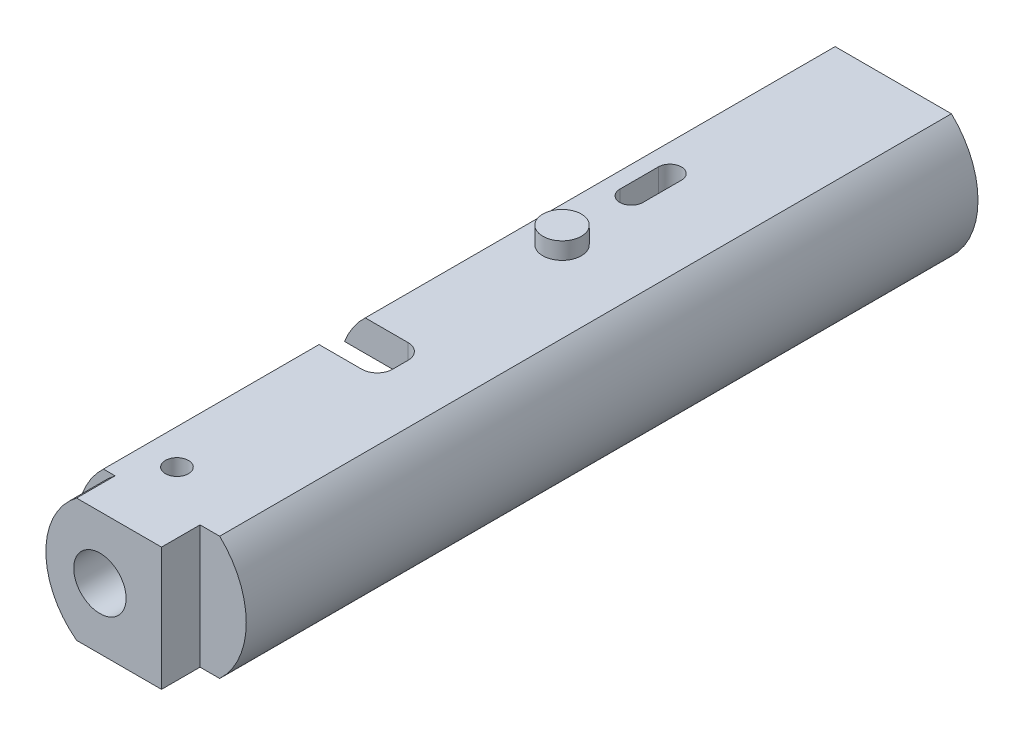
from build123d import *

# Parameters (mm, degrees)
SKETCH1_R                  = 11
BOSS_EXTRUDE1_DEPTH        = 100
CUT_EXTRUDE1_DEPTH         = 102.202766761
SKETCH3_R                  = 2
CUT_EXTRUDE2_DEPTH         = 60
CUT_EXTRUDE3_START         = -15
SKETCH4_W                  = 13.898015679
SKETCH4_H                  = 8
CUT_EXTRUDE3_DEPTH         = 65
CUT_EXTRUDE4_DEPTH         = 102.867561078
CUT_EXTRUDE4_DEPTH_BACK    = 102.867561078
SKETCH5_W                  = 12
SKETCH5_H                  = 10
M8_TAPPED_HOLE1_D          = 6.8
M8_TAPPED_HOLE1_DEPTH      = 10
M8_TAPPED_HOLE1_TIP        = 2.042926105
CUT_EXTRUDE5_START         = -3
SKETCH8_R                  = 1.5
CUT_EXTRUDE5_DEPTH         = 105.867561078
CUT_EXTRUDE6_DEPTH         = 102.867561078
CUT_EXTRUDE7_DEPTH         = 102.316336294
CUT_EXTRUDE7_DEPTH_BACK    = 102.316336294
M12X1_5_TAPPED_HOLE1_D     = 10.5
M12X1_5_TAPPED_HOLE1_DEPTH = 19.5
M12X1_5_TAPPED_HOLE1_TIP   = 3.15451825
SKETCH12_R                 = 2.5
BOSS_EXTRUDE2_DEPTH        = 2.2
BOSS_EXTRUDE3_START        = 2.2
SKETCH13_R                 = 2.5
BOSS_EXTRUDE3_DEPTH        = 2.2
SKETCH14_R                 = 3.5
CUT_EXTRUDE8_DEPTH         = 40
SKETCH15_R                 = 14.729549922
SKETCH15_R_2               = 10.018203868
CUT_EXTRUDE9_DEPTH         = 5


with BuildPart() as part:
    # Sketch1 → Boss-Extrude1 (new body)
    with BuildSketch(Plane.XY):
        Circle(SKETCH1_R)
    extrude(amount=BOSS_EXTRUDE1_DEPTH)

    # Sketch2 → Cut-Extrude1 (cut, through all)
    with BuildSketch(Plane.XY.offset(100)):
        with BuildLine():
            Line((-7.549834435, 8), (7.549834435, 8))
            ThreePointArc((7.549834435, 8), (0, 11), (-7.549834435, 8))
        make_face()
        with BuildLine():
            Line((-7.549834435, -8), (7.549834435, -8))
            ThreePointArc((7.549834435, -8), (0, -11), (-7.549834435, -8))
        make_face()
    extrude(amount=-CUT_EXTRUDE1_DEPTH, mode=Mode.SUBTRACT)

    # Sketch3 → Cut-Extrude2 (cut)
    with BuildSketch(Plane.XY.offset(100)):
        with Locations((-3, 0)):
            Circle(SKETCH3_R)
    extrude(amount=-CUT_EXTRUDE2_DEPTH, mode=Mode.SUBTRACT)

    # Sketch4 → Cut-Extrude3 (cut)
    with BuildSketch(Plane.XY.offset(100).offset(CUT_EXTRUDE3_START)):
        with Locations((-5.94900784, 0)):
            Rectangle(SKETCH4_W, SKETCH4_H)
    extrude(amount=-CUT_EXTRUDE3_DEPTH, mode=Mode.SUBTRACT)

    # Sketch5 → Cut-Extrude4 (cut, two sides: drawn at the far end of the back side and taken through both)
    with BuildSketch(Plane(origin=(0, -8, 0), x_dir=(-1, 0, 0), z_dir=(0, -1, 0)).offset(-CUT_EXTRUDE4_DEPTH_BACK)):
        with Locations((-11, -100)):
            Rectangle(SKETCH5_W, SKETCH5_H)
    extrude(amount=CUT_EXTRUDE4_DEPTH + CUT_EXTRUDE4_DEPTH_BACK, mode=Mode.SUBTRACT)

    # M8 Tapped Hole1
    with Locations(Plane(origin=(-3, -0.07100101, 100), x_dir=(1, 0, 0), z_dir=(0, 0, 1))):
        with Locations((0, 0)):
            Hole(M8_TAPPED_HOLE1_D / 2, depth=M8_TAPPED_HOLE1_DEPTH)
            with Locations((0, 0, -(M8_TAPPED_HOLE1_DEPTH + M8_TAPPED_HOLE1_TIP / 2))):  # 118° drill point
                Cone(0, M8_TAPPED_HOLE1_D / 2, M8_TAPPED_HOLE1_TIP, mode=Mode.SUBTRACT)

    # Sketch8 → Cut-Extrude5 (cut)
    with BuildSketch(Plane(origin=(0, -8, 0), x_dir=(-1, 0, 0), z_dir=(0, -1, 0)).offset(CUT_EXTRUDE5_START)):
        with Locations(Location((3, -90, 0), (0, 0, 270))):
            Circle(SKETCH8_R)
    cut_extrude5 = extrude(amount=CUT_EXTRUDE5_DEPTH, mode=Mode.SUBTRACT)

    # Mirror3: Cut-Extrude5 across plane
    add(cut_extrude5.mirror(Plane.ZX), mode=Mode.SUBTRACT)

    # Sketch9 → Cut-Extrude6 (cut, through all)
    with BuildSketch(Plane(origin=(0, -8, 0), x_dir=(-1, 0, 0), z_dir=(0, -1, 0))):
        with BuildLine():
            Line((2.5, -30), (2.5, -25))
            ThreePointArc((2.5, -25), (4, -23.5), (5.5, -25))
            Line((5.5, -25), (5.5, -30))
            ThreePointArc((5.5, -30), (4, -31.5), (2.5, -30))
        make_face()
    extrude(amount=-CUT_EXTRUDE6_DEPTH, mode=Mode.SUBTRACT)

    # Sketch10 → Cut-Extrude7 (cut, two sides: drawn at the far end of the back side and taken through both)
    with BuildSketch(Plane(origin=(0, 4, 0), x_dir=(-1, 0, 0), z_dir=(0, -1, 0)).offset(-CUT_EXTRUDE7_DEPTH_BACK)):
        with BuildLine():
            Line((2, -67), (19.82874578, -67))
            Line((19.82874578, -67), (19.82874578, -61))
            Line((19.82874578, -61), (2, -61))
            ThreePointArc((2, -61), (0.585786438, -61.585786438), (0, -63))
            Line((0, -63), (0, -65))
            ThreePointArc((0, -65), (0.585786438, -66.414213562), (2, -67))
        make_face()
    extrude(amount=CUT_EXTRUDE7_DEPTH + CUT_EXTRUDE7_DEPTH_BACK, mode=Mode.SUBTRACT)

    # M12x1.5 Tapped Hole1
    with Locations(Plane(origin=(0, 0, 0), x_dir=(-1, 0, 0), z_dir=(0, 0, -1))):
        with Locations((0, 0)):
            Hole(M12X1_5_TAPPED_HOLE1_D / 2, depth=M12X1_5_TAPPED_HOLE1_DEPTH)
            with Locations((0, 0, -(M12X1_5_TAPPED_HOLE1_DEPTH + M12X1_5_TAPPED_HOLE1_TIP / 2))):  # 118° drill point
                Cone(0, M12X1_5_TAPPED_HOLE1_D / 2, M12X1_5_TAPPED_HOLE1_TIP, mode=Mode.SUBTRACT)

    # Sketch12 → Boss-Extrude2 (add)
    with BuildSketch(Plane.XZ.offset(8)):
        with Locations(Location((-3, 40, 0), (0, 0, 90))):
            Circle(SKETCH12_R)
    extrude(amount=BOSS_EXTRUDE2_DEPTH)

    # Sketch13 → Boss-Extrude3 (add)
    with BuildSketch(Plane(origin=(0, 8, 0), x_dir=(1, 0, 0), z_dir=(0, 1, 0)).offset(BOSS_EXTRUDE3_START)):
        with Locations(Location((-3, -40, 0), (0, 0, 270))):
            Circle(SKETCH13_R)
    extrude(amount=-BOSS_EXTRUDE3_DEPTH)

    # Sketch14 → Cut-Extrude8 (cut)
    with BuildSketch(Plane(origin=(0, 0, 0), x_dir=(-1, 0, 0), z_dir=(0, 0, -1))):
        Circle(SKETCH14_R)
    extrude(amount=-CUT_EXTRUDE8_DEPTH, mode=Mode.SUBTRACT)

    # Sketch15 → Cut-Extrude9 (cut)
    with BuildSketch(Plane.XY.offset(100)):
        Circle(SKETCH15_R)
        Circle(SKETCH15_R_2, mode=Mode.SUBTRACT)
    extrude(amount=-CUT_EXTRUDE9_DEPTH, mode=Mode.SUBTRACT)


solid = part.part
